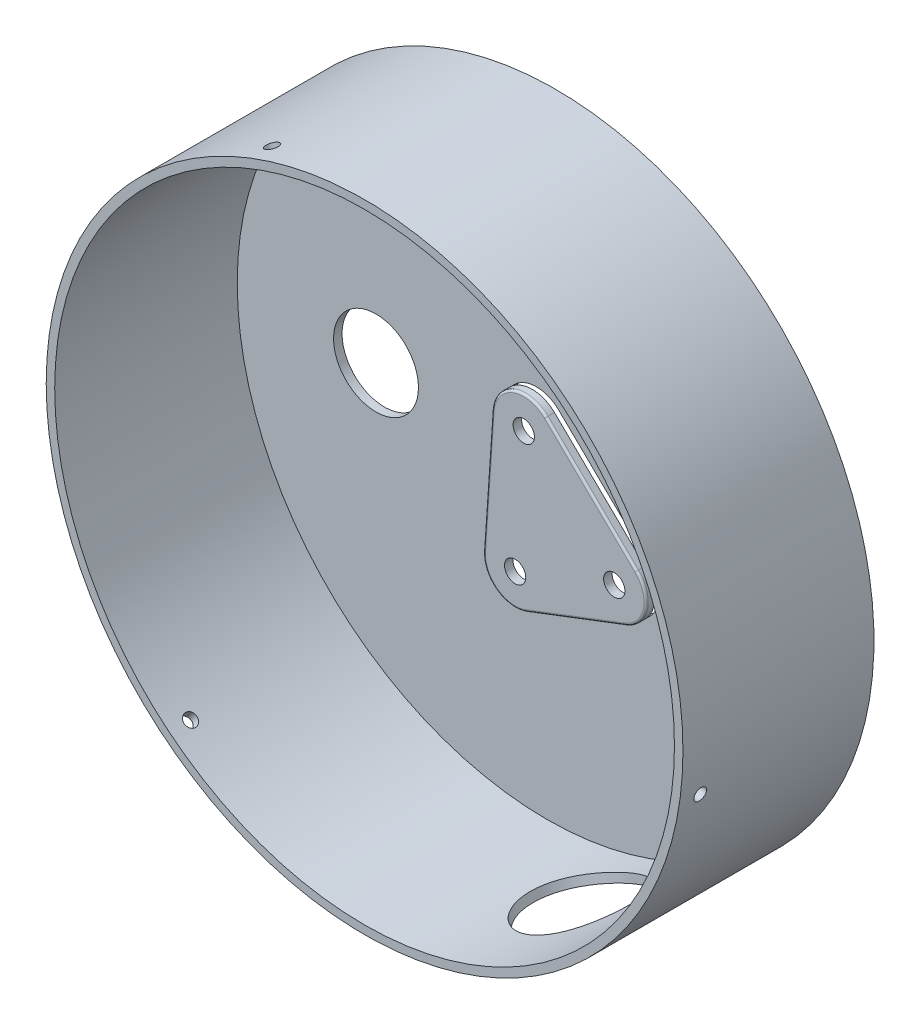
SolidWorks part; units mm, degrees
ref_plane "Front plane" through (0, 0, 0) normal (0, 0, 1) x (1, 0, 0)
ref_plane "Top plane" through (0, 0, 0) normal (0, 1, 0) x (1, 0, 0)
ref_plane "Right plane" through (0, 0, 0) normal (1, 0, 0) x (0, 0, -1)
sketch "Sketch 1" plane through (0, 0, 0) normal (0, 0, 1) x (1, 0, 0)
  circle A0 centre (0, 0) radius 75
  circle A1 centre (0, 0) radius 73
  dimension "D1" = 150
  dimension "D2" = 146
extrude "Boss-Extrude 1" add sketch "Sketch 1" along normal blind 48
sketch "Sketch 2" plane through (0, 0, 0) normal (0, 0, 1) x (1, 0, 0)
  circle A0 centre (0, 0) radius 75 construction
  circle A1 centre (0, 0) radius 75
  point P4 (0, 0)
extrude "Boss-Extrude 2" add sketch "Sketch 2" along normal blind 5
sketch "Sketch 4" plane through (0, 0, 0) normal (0, 0, 1) x (1, 0, 0)
  circle A0 centre (-40.31, 0) radius 10
  circle A1 centre (0, 0) radius 73 construction
  dimension "D1" = 20
  dimension "D2" = 40.31
extrude "Cut-Extrude 8" cut sketch "Sketch 4" along normal through all
sketch "Sketch 8" plane through (0, 0, 0) normal (0, 0, -1) x (-1, 0, 0)
  line L0 (-0.2433, -0.636) -> (5.8919, 15.4007) construction
  line L1 (12.0122, -22.6315) -> (9.9838, 7.0493)
  line L2 (-2.7293, 11.9129) -> (-24.0504, -8.8349)
  line L3 (-21.4998, -21.2148) -> (1.8498, -30.1478)
  arc A1 (9.9838, 7.0493) -> (-2.7293, 11.9129) centre (2.5012, 6.5379) ccw
  arc A2 (-21.4998, -21.2148) -> (-24.0504, -8.8349) centre (-18.8199, -14.21) cw
  arc A3 (1.8498, -30.1478) -> (12.0122, -22.6315) centre (4.5297, -23.1429) ccw
  circle A5 centre (0, 0) radius 75 construction
  circle A7 centre (0, 0) radius 75
  point P0 (-9.825, -25.6813)
  dimension "D1" = 7.5
  dimension "D2" = 7.5
  dimension "D3" = 7.5
  dimension "D4" = 29.75
  dimension "D7" = 7
  dimension "D5" = 12.5
  dimension "D6" = 12.5
extrude "Cut-Extrude 10" cut sketch "Sketch 8" against normal blind 3
ref_plane "Reference plane 1" through (26.7987, -70.0488, 0) normal (0.3573, -0.934, 0) x (-0.934, -0.3573, 0)
sketch "Sketch 11" plane through (26.7987, -70.0488, 0) normal (0.3573, -0.934, 0) x (-0.934, -0.3573, 0)
  line L2 (-75, -48) -> (75, -48) construction
  circle A0 centre (0, -23) radius 12.5
  dimension "D2" = 25
  dimension "D1" = 25
extrude "Cut-Extrude 12" cut sketch "Sketch 11" against normal up to next
sketch "Sketch 12" plane through (0, 0, 5) normal (0, 0, 1) x (1, 0, 0)
  circle A1 centre (0, 0) radius 73
  circle A2 centre (0, 0) radius 73
  dimension "D1" = 0
ref_plane "Reference plane 2" through (74.8255, -5.1138, 0) normal (0.9977, -0.0682, 0) x (0, 0, -1)
ref_plane "Reference plane 3" through (-26.7987, 70.0488, 0) normal (-0.3573, 0.934, 0) x (0.934, 0.3573, 0)
ref_plane "Reference plane 4" through (-52.3055, -53.7507, 0) normal (-0.6974, -0.7167, 0) x (-0.7167, 0.6974, 0)
sketch "Sketch 20" plane through (0, 0, 0) normal (0, 0, -1) x (-1, 0, 0)
  line L3 (-2.7293, 11.9129) -> (-24.0504, -8.8349)
  line L4 (-21.4998, -21.2148) -> (1.8498, -30.1478)
  line L5 (12.0122, -22.6315) -> (9.9838, 7.0493)
  line L6 (-2.7293, 11.9129) -> (-24.0504, -8.8349)
  line L7 (-21.4998, -21.2148) -> (1.8498, -30.1478)
  line L8 (12.0122, -22.6315) -> (9.9838, 7.0493)
  circle A0 centre (2.5012, 6.5379) radius 2.5
  circle A1 centre (4.5297, -23.1429) radius 2.5
  circle A2 centre (-18.8199, -14.21) radius 2.5
  arc A3 (9.9838, 7.0493) -> (-2.7293, 11.9129) centre (2.5012, 6.5379) ccw
  arc A4 (-24.0504, -8.8349) -> (-21.4998, -21.2148) centre (-18.8199, -14.21) ccw
  arc A5 (1.8498, -30.1478) -> (12.0122, -22.6315) centre (4.5297, -23.1429) ccw
  arc A6 (9.9838, 7.0493) -> (-2.7293, 11.9129) centre (2.5012, 6.5379) ccw
  arc A7 (-24.0504, -8.8349) -> (-21.4998, -21.2148) centre (-18.8199, -14.21) ccw
  arc A8 (1.8498, -30.1478) -> (12.0122, -22.6315) centre (4.5297, -23.1429) ccw
  dimension "D2" = 5
  dimension "D3" = 5
  dimension "D4" = 5
  dimension "D1" = 0
extrude "Cut-Extrude 19" cut sketch "Sketch 20" against normal through all contours A0 | A2 | A1
sketch "Sketch 21" plane through (0, 0, 5) normal (0, 0, 1) x (1, 0, 0)
  line L3 (24.0504, -8.8349) -> (2.7293, 11.9129)
  line L4 (-1.8498, -30.1478) -> (21.4998, -21.2148)
  line L5 (-9.9838, 7.0493) -> (-12.0122, -22.6315)
  line L6 (24.0504, -8.8349) -> (2.7293, 11.9129)
  line L7 (-1.8498, -30.1478) -> (21.4998, -21.2148)
  line L8 (-9.9838, 7.0493) -> (-12.0122, -22.6315)
  circle A0 centre (-4.5297, -23.1429) radius 2.5 construction
  circle A1 centre (18.8199, -14.21) radius 2.5 construction
  circle A3 centre (-2.5012, 6.5379) radius 2.5 construction
  arc A4 (2.7293, 11.9129) -> (-9.9838, 7.0493) centre (-2.5012, 6.5379) ccw
  arc A5 (21.4998, -21.2148) -> (24.0504, -8.8349) centre (18.8199, -14.21) ccw
  arc A6 (-12.0122, -22.6315) -> (-1.8498, -30.1478) centre (-4.5297, -23.1429) ccw
  arc A7 (2.7293, 11.9129) -> (-9.9838, 7.0493) centre (-2.5012, 6.5379) ccw
  arc A8 (21.4998, -21.2148) -> (24.0504, -8.8349) centre (18.8199, -14.21) ccw
  arc A9 (-12.0122, -22.6315) -> (-1.8498, -30.1478) centre (-4.5297, -23.1429) ccw
  circle A10 centre (-4.5297, -23.1429) radius 2.5
  circle A11 centre (18.8199, -14.21) radius 2.5
  circle A12 centre (-2.5012, 6.5379) radius 2.5
  dimension "D1" = 0
extrude "Boss-Extrude 3" add sketch "Sketch 21" along normal blind 3 contours A7 L8 A9 L7 A8 L6 | A11 | A10 | A12
sketch "Sketch 22" plane through (0, 0, 0) normal (0, 0, -1) x (-1, 0, 0)
  line L3 (-2.7293, 11.9129) -> (-24.0504, -8.8349)
  line L4 (-21.4998, -21.2148) -> (1.8498, -30.1478)
  line L5 (12.0122, -22.6315) -> (9.9838, 7.0493)
  line L6 (-2.7293, 11.9129) -> (-24.0504, -8.8349)
  line L7 (-21.4998, -21.2148) -> (1.8498, -30.1478)
  line L8 (12.0122, -22.6315) -> (9.9838, 7.0493)
  arc A3 (9.9838, 7.0493) -> (-2.7293, 11.9129) centre (2.5012, 6.5379) ccw
  arc A4 (-24.0504, -8.8349) -> (-21.4998, -21.2148) centre (-18.8199, -14.21) ccw
  arc A5 (1.8498, -30.1478) -> (12.0122, -22.6315) centre (4.5297, -23.1429) ccw
  arc A6 (9.9838, 7.0493) -> (-2.7293, 11.9129) centre (2.5012, 6.5379) ccw
  arc A7 (-24.0504, -8.8349) -> (-21.4998, -21.2148) centre (-18.8199, -14.21) ccw
  arc A8 (1.8498, -30.1478) -> (12.0122, -22.6315) centre (4.5297, -23.1429) ccw
  dimension "D1" = 0
extrude "Cut-Extrude 21" cut sketch "Sketch 22" against normal blind 6 contours A6 L6 A7 L7 A8 L8
fillet "Fillet 2" radius 0.5 6 edges at (-10.998, -7.7911, 8) (-5.1811, 13.5428, 8) (13.3899, 1.539, 8) (26.1656, -15.7234, 8) (9.825, -25.6813, 8) (-8.9895, -29.1728, 8)
sketch "Sketch 23" plane through (0, 0, 8) normal (0, 0, 1) x (1, 0, 0)
  line L0 (0, 0) -> (-2.5012, 6.5379)
  line L1 (-2.5012, 6.5379) -> (-30.7915, 80.4852) construction
  line L3 (-9.4849, 7.0152) -> (-11.5134, -22.6656)
  line L4 (-2.0285, -29.6808) -> (21.3211, -20.7479)
  line L5 (23.7017, -9.1932) -> (2.3806, 11.5546)
  line L6 (-9.4849, 7.0152) -> (-11.5134, -22.6656)
  line L7 (-2.0285, -29.6808) -> (21.3211, -20.7479)
  line L8 (23.7017, -9.1932) -> (2.3806, 11.5546)
  arc A3 (2.3806, 11.5546) -> (-9.4849, 7.0152) centre (-2.5012, 6.5379) ccw
  arc A4 (-11.5134, -22.6656) -> (-2.0285, -29.6808) centre (-4.5297, -23.1429) ccw
  arc A5 (21.3211, -20.7479) -> (23.7017, -9.1932) centre (18.8199, -14.21) ccw
  arc A6 (2.3806, 11.5546) -> (-9.4849, 7.0152) centre (-2.5012, 6.5379) ccw
  arc A7 (-11.5134, -22.6656) -> (-2.0285, -29.6808) centre (-4.5297, -23.1429) ccw
  arc A8 (21.3211, -20.7479) -> (23.7017, -9.1932) centre (18.8199, -14.21) ccw
  dimension "D1" = 0
ref_plane "Reference plane 5" through (-26.7987, 70.0488, 0) normal (-0.3573, 0.934, 0) x (0.934, 0.3573, 0)
sketch "Sketch 24" plane through (-26.7987, 70.0488, 0) normal (-0.3573, 0.934, 0) x (0.934, 0.3573, 0)
  line L0 (0, -23) -> (0, -54.126) construction
  line L1 (-75, -48) -> (75, -48) construction
  circle A0 centre (0, -23) radius 12.5 construction
  circle A2 centre (0, -43) radius 1.5
  dimension "D1" = 3
  dimension "D2" = 5
extrude "Cut-Extrude 22" cut sketch "Sketch 24" against normal up to next
ref_plane "Reference plane 6" through (0, 0, 0) normal (0.934, 0.3573, 0) x (0, 0, -1)
sketch "Sketch 25" plane through (0, 0, 0) normal (0.934, 0.3573, 0) x (0, 0, -1)
  line L0 (0, 0) -> (-14.4445, 0) construction
pattern_circular "Circular pattern 1" count 3 over 360 about axis through (0, 0, 0) along (0, 0, 1) of "Cut-Extrude 22"
